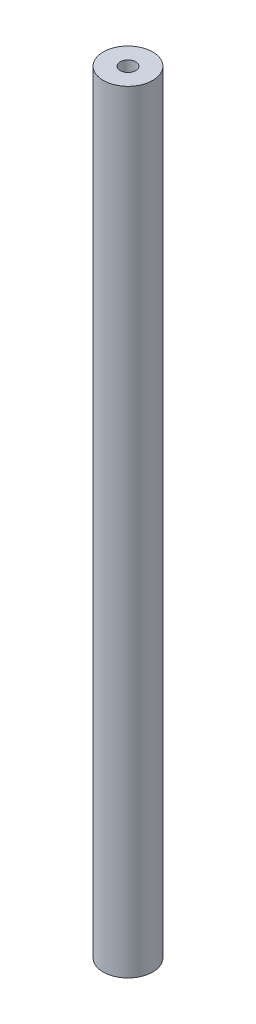
SolidWorks part; units mm, degrees
material "S45C"
ref_plane "前视基准面" through (0, 0, 0) normal (0, 0, 1) x (1, 0, 0)
ref_plane "上视基准面" through (0, 0, 0) normal (0, 1, 0) x (1, 0, 0)
ref_plane "右视基准面" through (0, 0, 0) normal (1, 0, 0) x (0, 0, -1)
sketch "草图1" plane through (0, 0, 0) normal (0, 1, 0) x (1, 0, 0)
  circle A0 centre (0, 0) radius 8
  dimension "D1" = 16
extrude "凸台-拉伸1" add sketch "草图1" along normal blind 250
hole_wizard "M6 螺纹孔1" positions "草图2" profile "草图3" tap size "M6" standard "GB"
sketch "草图2" plane through (0, 250, 0) normal (0, 1, 0) x (1, 0, 0)
  point P0 (0, 0)
sketch "草图3" plane through (0, 250, 0) normal (1, 0, 0) x (0, 0, 1)
  line L0 (0, 0) -> (0, 16.5022)
  line L1 (0, 16.5022) -> (2.5, 15)
  line L2 (2.5, 15) -> (2.5, 0)
  line L5 (2.5, 0) -> (0, 0)
  line L10 (0, 16.5022) -> (-2.5, 15) construction
  line L11 (0, -6.35) -> (0, 107.95) construction
  dimension "螺纹孔钻头直径" = 5
  dimension "螺纹孔钻头深度" = 15
  dimension "导头角度" = 118
cosmetic thread "孔螺蚊线1" parameters "D1"=12, "D2"=6
